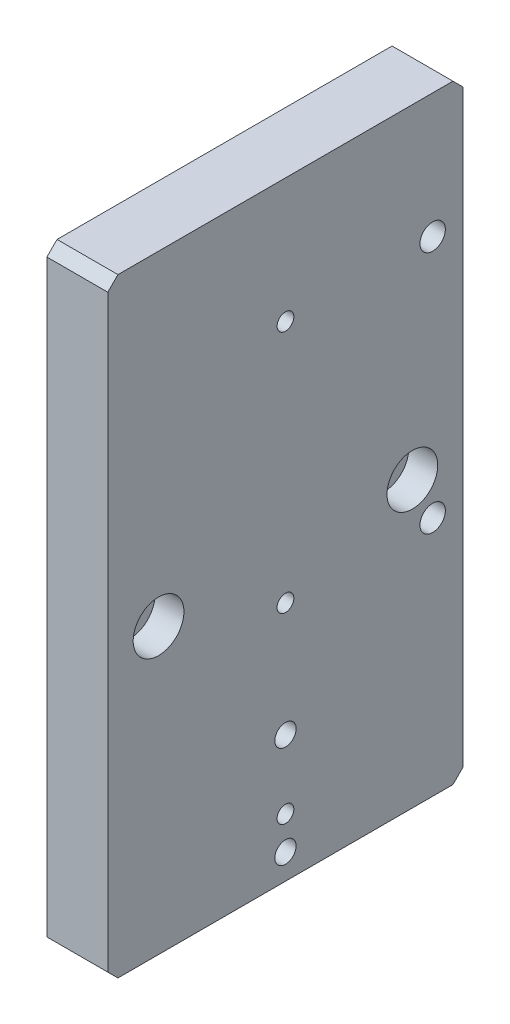
SolidWorks part; units mm, degrees
material "AL6061"
ref_plane "Front Plane" through (0, 0, 0) normal (0, 0, 1) x (1, 0, 0)
ref_plane "Top Plane" through (0, 0, 0) normal (0, 1, 0) x (1, 0, 0)
ref_plane "Right Plane" through (0, 0, 0) normal (1, 0, 0) x (0, 0, -1)
sketch "Sketch1" plane through (0, 0, 0) normal (1, 0, 0) x (0, 0, -1)
  line L1 (-35, -60) -> (35, -60)
  line L2 (-35, -60) -> (-35, 60)
  line L3 (-35, 60) -> (35, 60)
  line L4 (35, -60) -> (35, 60)
  line L5 (-35, -60) -> (35, 60) construction
  line L6 (-35, 60) -> (35, -60) construction
  point P0 (0, 0)
  dimension "D1" = 70
  dimension "D2" = 120
extrude "Boss-Extrude1" add sketch "Sketch1" along normal blind 12
hole_wizard "M5 Tapped Hole1" positions "Sketch2" profile "Sketch3" tap size "M5" standard "GB"
sketch "Sketch2" plane through (0, 0, 0) normal (-1, 0, 0) x (0, 0, 1)
  point P0 (0, -35)
  point P3 (0, -55)
sketch "Sketch3" plane through (0, -35, 0) normal (0, 1, 0) x (0, 0, 1)
  line L0 (0, 0) -> (0, 13.6618)
  line L1 (0, 13.6618) -> (2.1, 12.4)
  line L2 (2.1, 12.4) -> (2.1, 0)
  line L5 (2.1, 0) -> (0, 0)
  line L10 (0, 13.6618) -> (-2.1, 12.4) construction
  line L11 (0, -6.35) -> (0, 107.95) construction
  dimension "螺纹孔钻头直径" = 4.2
  dimension "螺纹孔钻头深度" = 12.4
  dimension "导头角度" = 118
cosmetic thread "Cosmetic Thread1" parameters "D1"=10, "D2"=5
cosmetic thread "Cosmetic Thread2" parameters "D1"=10, "D2"=5
hole_wizard "CBORE for M5 Hexagon socket head cap screws1" positions "Sketch4" profile "Sketch5" counterbore size "M5" standard "GB" end condition through all
sketch "Sketch4" plane through (12, 0, 0) normal (1, 0, 0) x (0, 0, -1)
  point P0 (25, -4)
  point P3 (-25, -4)
sketch "Sketch5" plane through (12, -4, -25) normal (0, 1, 0) x (0, 0, -1)
  line L0 (0, 0) -> (0, 12)
  line L1 (0, 12) -> (2.75, 12)
  line L3 (2.75, 12) -> (2.75, 5.7)
  line L4 (2.75, 5.7) -> (5, 5.7)
  line L5 (5, 5.7) -> (5, 0)
  line L7 (5, 0) -> (0, 0)
  line L11 (0, -6.35) -> (0, 107.95) construction
  dimension "通孔孔直径" = 5.5
  dimension "通孔孔深度" = 12
  dimension "柱形沉头孔直径" = 10
  dimension "柱形沉头孔深度" = 5.7
hole_wizard "M4 Tapped Hole1" positions "Sketch6" profile "Sketch7" tap size "M4" standard "GB"
sketch "Sketch6" plane through (12, 0, 0) normal (1, 0, 0) x (0, 0, -1)
  point P0 (0, -48.5)
  point P3 (0, -12.5)
  point P6 (0, 35.5)
sketch "Sketch7" plane through (12, -48.5, 0) normal (0, 1, 0) x (0, 0, -1)
  line L0 (0, 0) -> (0, 11.0914)
  line L1 (0, 11.0914) -> (1.65, 10.1)
  line L2 (1.65, 10.1) -> (1.65, 0)
  line L5 (1.65, 0) -> (0, 0)
  line L10 (0, 11.0914) -> (-1.65, 10.1) construction
  line L11 (0, -6.35) -> (0, 107.95) construction
  dimension "螺纹孔钻头直径" = 3.3
  dimension "螺纹孔钻头深度" = 10.1
  dimension "导头角度" = 118
cosmetic thread "Cosmetic Thread3" parameters "D1"=8, "D2"=4
cosmetic thread "Cosmetic Thread4" parameters "D1"=8, "D2"=4
cosmetic thread "Cosmetic Thread5" parameters "D1"=8, "D2"=4
hole_wizard "Ø5.0mm Dowel Hole1" positions "Sketch8" profile "Sketch9" hole size "Ø5.0" standard "GB"
sketch "Sketch8" plane through (12, 0, 0) normal (1, 0, 0) x (0, 0, -1)
  line L0 (29, -12) -> (29, -13) construction
  point P0 (29, 35.5)
  point P9 (29, -12.5)
sketch "Sketch9" plane through (12, 35.5, -29) normal (0, 1, 0) x (0, 0, -1)
  line L0 (0, 0) -> (0, 9.5022)
  line L1 (0, 9.5022) -> (2.5, 8)
  line L2 (2.5, 8) -> (2.5, 0)
  line L5 (2.5, 0) -> (0, 0)
  line L10 (0, 9.5022) -> (-2.5, 8) construction
  line L11 (0, -6.35) -> (0, 107.95) construction
  dimension "孔直径" = 5
  dimension "孔深度" = 8
  dimension "导头角度" = 118
chamfer "Chamfer1" distance 2 angle 45 4 edges at (6, -60, -35) (6, -60, 35) (6, 60, -35) (6, 60, 35)
